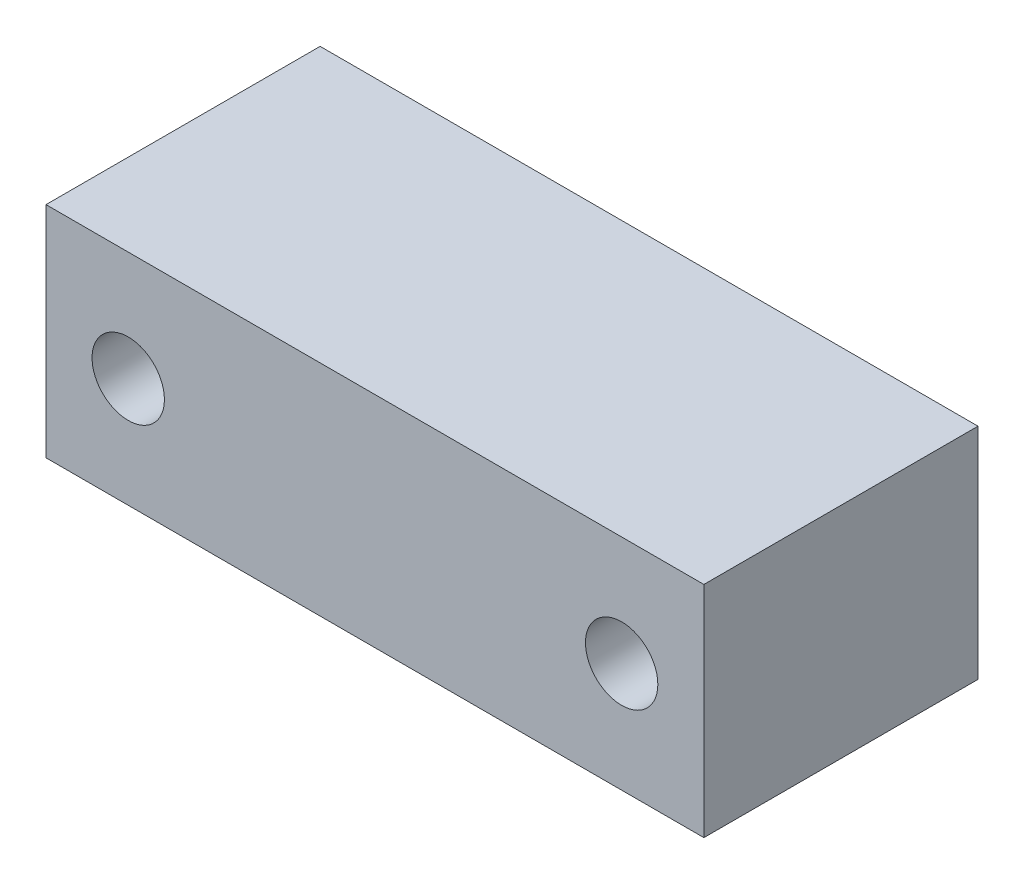
from build123d import *

# Parameters (mm, degrees)
SKETCH_1_W         = 60
SKETCH_1_H         = 20
EXTRUDE_1_DEPTH    = 25
HOLE_WIZARD_M6_1_D = 6.6


with BuildPart() as part:
    # 草图1 → 凸台-拉伸1 (new body)
    with BuildSketch(Plane.XY):
        Rectangle(SKETCH_1_W, SKETCH_1_H)
    extrude(amount=EXTRUDE_1_DEPTH)

    # M6 间隙孔1 (through all)
    with Locations(Plane.XY.offset(25)):
        with Locations((-22.5, 0), (22.5, 0)):
            Hole(HOLE_WIZARD_M6_1_D / 2)


solid = part.part
